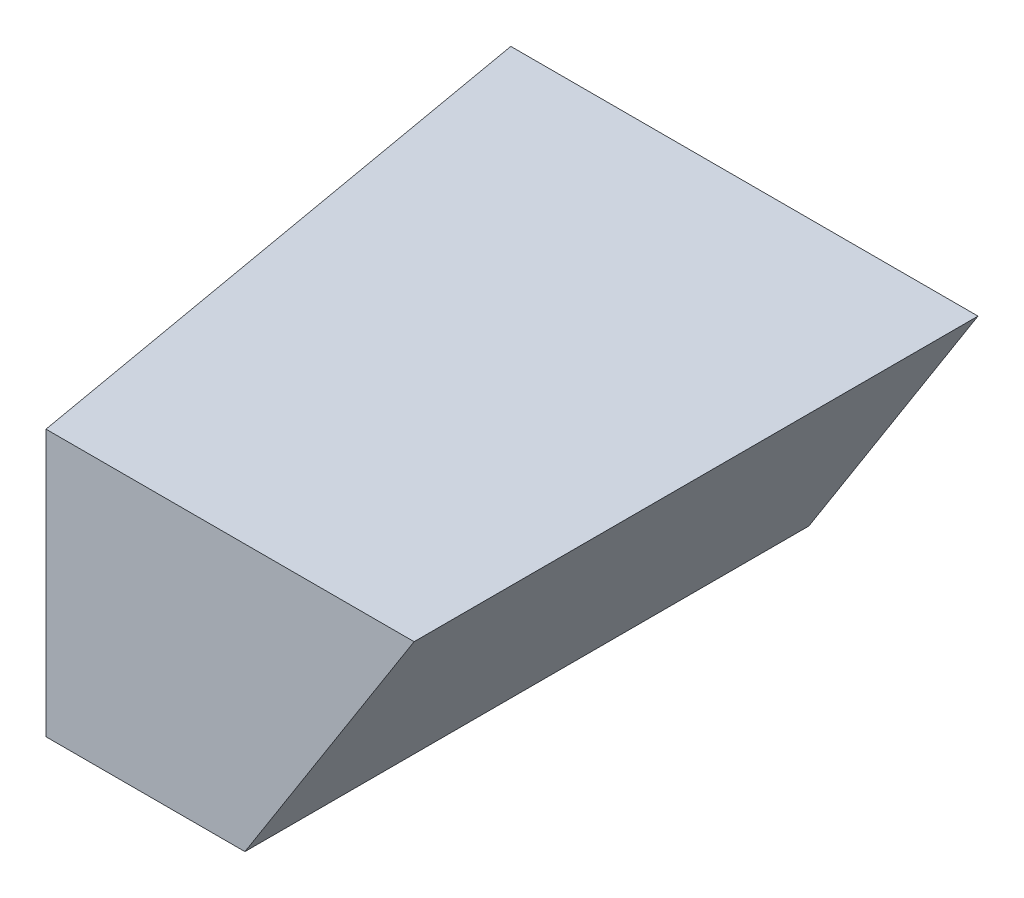
SolidWorks part; units mm, degrees
ref_plane "前视基准面" through (0, 0, 0) normal (0, 0, 1) x (1, 0, 0)
ref_plane "上视基准面" through (0, 0, 0) normal (0, 1, 0) x (1, 0, 0)
ref_plane "右视基准面" through (0, 0, 0) normal (1, 0, 0) x (0, 0, -1)
sketch "草图1" plane through (0, 0, 0) normal (0, 0, 1) x (1, 0, 0)
  line L3 (-4.4079, 5) -> (-7.4079, 5)
  line L4 (-7.4079, 5) -> (-7.4079, 6.5)
  line L6 (-7.4079, 6.5) -> (-3.4554, 6.5)
  line L13 (-3.4554, 6.5) -> (-4.4079, 5)
  dimension "D1" = 3
  dimension "D2" = 0.9525
  dimension "D3" = 1.5
extrude "凸台-拉伸1" add sketch "草图1" along normal blind 3.175 contours L4 L6 L13 L3
sketch "草图3" plane through (0, 5, 0) normal (0, -1, 0) x (1, 0, 0)
  line L0 (-7.4079, 0) -> (-6.0859, 0)
  line L1 (-4.4079, 0) -> (-7.4079, 0) construction
  line L2 (-7.4079, 0) -> (-7.4079, 3.175)
  line L3 (-7.4079, 3.175) -> (-5.5279, 3.175)
  line L4 (-4.4079, 3.175) -> (-7.4079, 3.175) construction
  line L5 (-6.0859, 0) -> (-5.5279, 3.175)
  dimension "D1" = 1.322
  dimension "D2" = 1.88
extrude "切除-拉伸1" cut sketch "草图3" against normal blind 3.175
